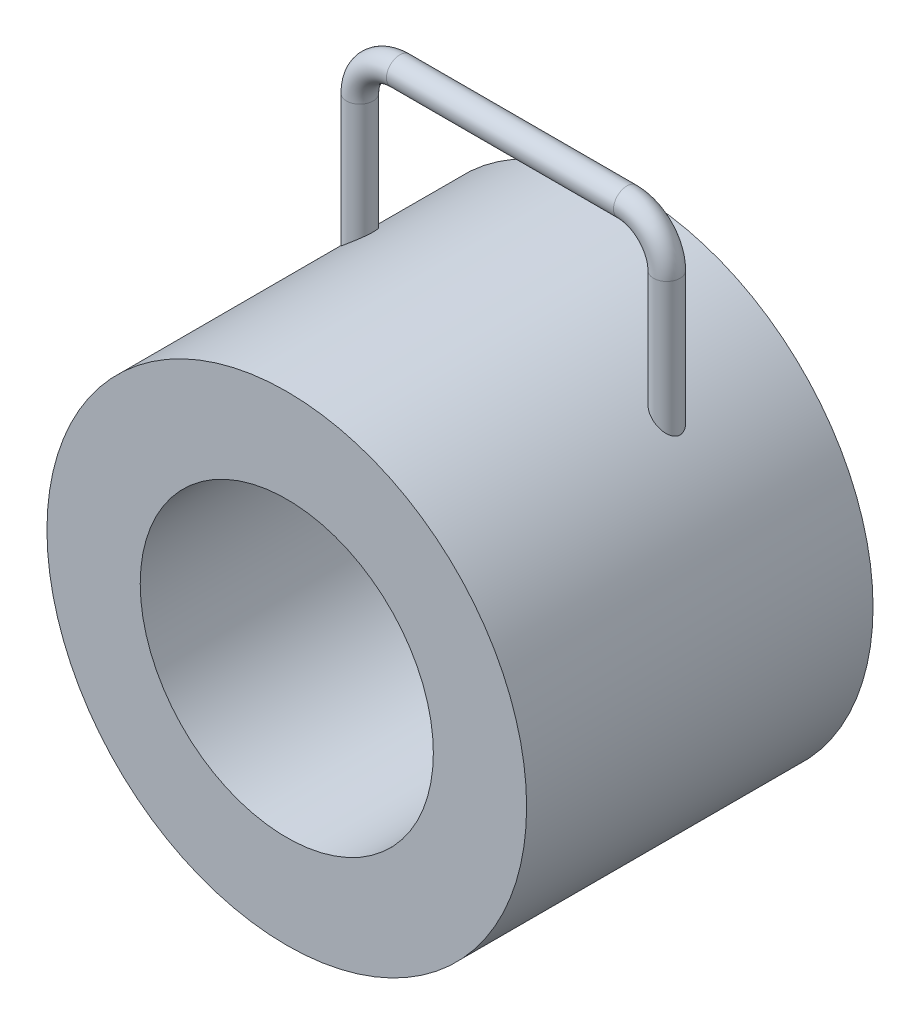
from build123d import *

# Parameters (mm, degrees)
SKETCH1_R           = 90
BOSS_EXTRUDE1_DEPTH = 130
SKETCH2_R           = 55
CUT_EXTRUDE1_DEPTH  = 100
SWEEP1_PROFILE_R    = 5


with BuildPart() as part:
    # Sketch1 → Boss-Extrude1 (new body)
    with BuildSketch(Plane.XY):
        Circle(SKETCH1_R)
    extrude(amount=BOSS_EXTRUDE1_DEPTH)

    # Sketch2 → Cut-Extrude1 (cut)
    with BuildSketch(Plane.XY.offset(130)):
        Circle(SKETCH2_R)
    extrude(amount=-CUT_EXTRUDE1_DEPTH, mode=Mode.SUBTRACT)

    # Sweep1: sweep along a path in Sketch3
    with BuildLine(Plane(origin=(0, 0, 45), x_dir=(-1, 0, 0), z_dir=(0, 0, -1))) as sweep1_path:
        Line((-57.6, 56.789164475), (-57.6, 115.589164475))
        ThreePointArc((-57.6, 115.589164475), (-53.206601718, 126.195766193), (-42.6, 130.589164475))
        Line((-42.6, 130.589164475), (42.6, 130.589164475))
        ThreePointArc((42.6, 130.589164475), (53.206601718, 126.195766193), (57.6, 115.589164475))
        Line((57.6, 115.589164475), (57.6, 56.789164475))
    # Sweep1 profile (on start of the path) → Sweep1 (sweep)
    with BuildSketch(Plane(origin=(57.6, 56.789164475, 45), x_dir=(0, 0, 1), z_dir=(0, 1, 0))):
        Circle(SWEEP1_PROFILE_R)
    sweep(path=sweep1_path.line)


solid = part.part
